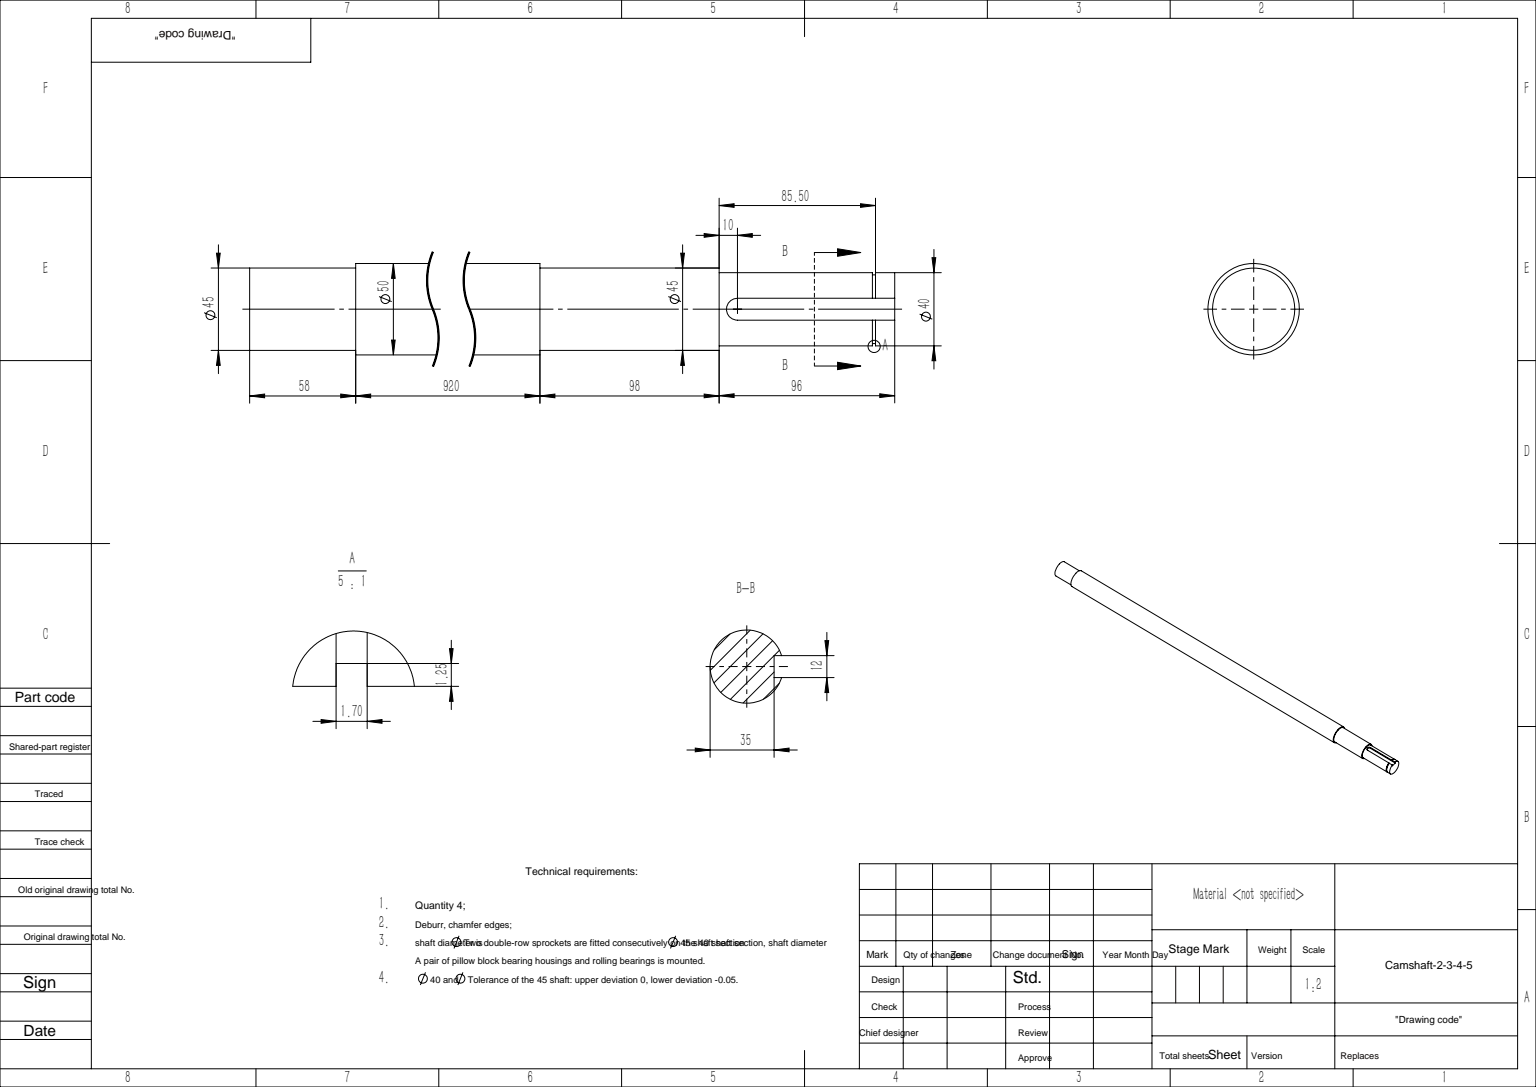
from build123d import *

# Parameters (mm, degrees)
CUT_EXTRUDE_1_DEPTH = 5
SKETCH_3_R          = 20
SKETCH_3_R_2        = 18.75
CUT_EXTRUDE_2_DEPTH = 1.7


with BuildPart() as part:
    # 草图1 → 旋转1 (revolve)
    with BuildSketch(Plane.XY):
        Polygon((0, 0), (0, 22.5), (58, 22.5), (58, 25), (978, 25), (978, 22.5), (1076, 22.5), (1076, 20), (1172, 20), (1172, 0), align=None)
    revolve(axis=Axis((1172, 0, 0), (-1, 0, 0)))

    # 草图2 → 切除-拉伸1 (cut)
    with BuildSketch(Plane(origin=(0, 20, 0), x_dir=(1, 0, 0), z_dir=(0, 1, 0))):
        with BuildLine():
            Line((1086, 6), (1182, 6))
            Line((1182, 6), (1182, -6))
            Line((1182, -6), (1086, -6))
            ThreePointArc((1086, -6), (1080, 0), (1086, 6))
        make_face()
    extrude(amount=-CUT_EXTRUDE_1_DEPTH, mode=Mode.SUBTRACT)

    # 草图3 → 切除-拉伸2 (cut)
    with BuildSketch(Plane(origin=(1161.5, 0, 0), x_dir=(0, 0, -1), z_dir=(1, 0, 0))):
        with Locations(Location((0, 0, 0), (0, 0, 90))):
            Circle(SKETCH_3_R)
        Circle(SKETCH_3_R_2, mode=Mode.SUBTRACT)
    extrude(amount=-CUT_EXTRUDE_2_DEPTH, mode=Mode.SUBTRACT)


solid = part.part
